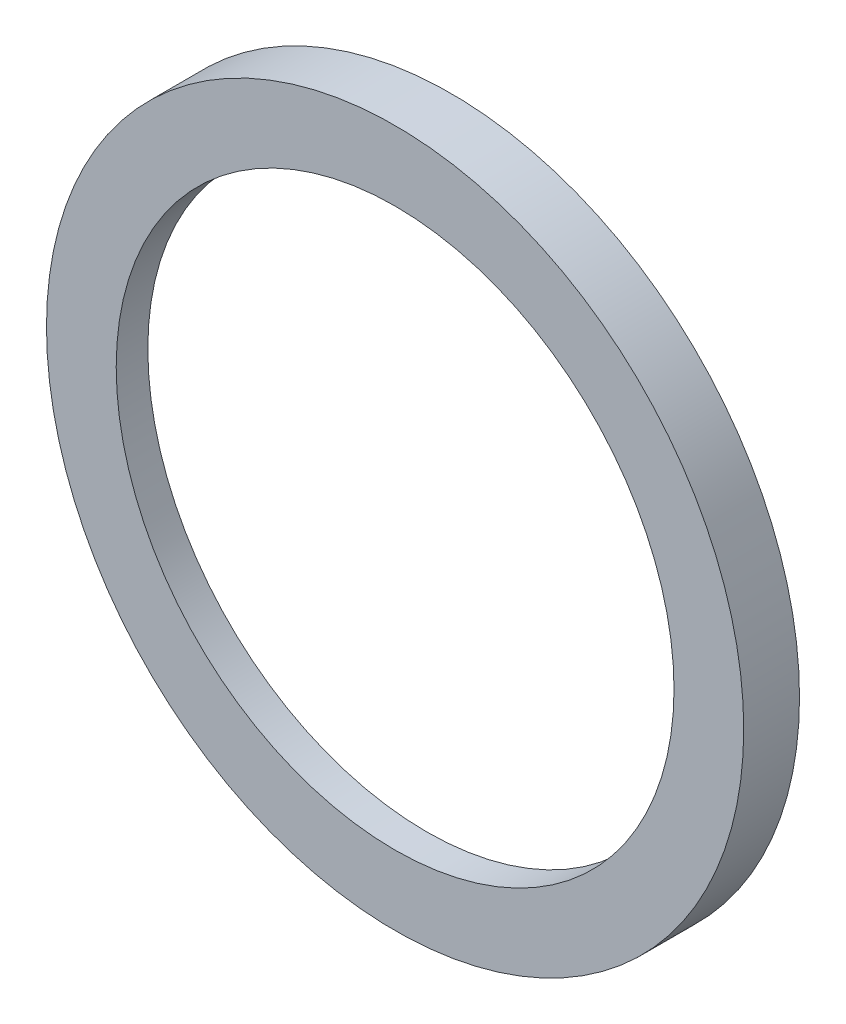
SolidWorks part; units mm, degrees
material "Q235"
ref_plane "Front Plane" through (0, 0, 0) normal (0, 0, 1) x (1, 0, 0)
ref_plane "Top Plane" through (0, 0, 0) normal (0, 1, 0) x (1, 0, 0)
ref_plane "Right Plane" through (0, 0, 0) normal (1, 0, 0) x (0, 0, -1)
sketch "Sketch1" plane through (0, 0, 0) normal (1, 0, 0) x (0, 0, -1)
  line L0 (0, 0) -> (30, 0) construction
  line L1 (0, 150) -> (0, 187.5)
  line L2 (0, 187.5) -> (30, 187.5)
  line L3 (30, 187.5) -> (30, 176)
  line L4 (30, 176) -> (17, 176)
  line L5 (17, 176) -> (17, 150)
  line L6 (17, 150) -> (0, 150)
  dimension "D1" = 30
  dimension "D2" = 13
  dimension "D3" = 375
  dimension "D4" = 352
  dimension "D5" = 300
revolve "Revolve1" add sketch "Sketch1" angle 360 about L0
hole_wizard "M8 Tapped Hole1" positions "Sketch3" profile "Sketch4" tap size "M8" standard "GB"
sketch "Sketch3" plane through (0, 0, -17) normal (0, 0, -1) x (-1, 0, 0)
  point P0 (0, 162.5)
  point P10 (95.5151, 131.4653)
  point P11 (154.5467, 50.2153)
  point P12 (154.5467, -50.2153)
  point P13 (95.5151, -131.4653)
  point P14 (0, -162.5)
  point P15 (-95.5151, -131.4653)
  point P16 (-154.5467, -50.2153)
  point P17 (-154.5467, 50.2153)
  point P18 (-95.5151, 131.4653)
  dimension "D1" = 162.5
  dimension "D2" = 10
sketch "Sketch4" plane through (0, 162.5, -17) normal (1, 0, 0) x (0, 1, 0)
  line L0 (0, 0) -> (0, 13)
  line L1 (0, 13) -> (3.4, 10.9571)
  line L2 (3.4, 10.9571) -> (3.4, 0)
  line L5 (3.4, 0) -> (0, 0)
  line L10 (0, 13) -> (-3.4, 10.9571) construction
  line L11 (0, -6.35) -> (0, 107.95) construction
  dimension "螺纹孔钻头直径" = 6.8
  dimension "螺纹孔钻头深度" = 13
  dimension "导头角度" = 118
cosmetic thread "Hole Cosmetic Thread1" parameters "D1"=10, "D2"=8
cosmetic thread "Hole Cosmetic Thread2" parameters "D1"=10, "D2"=8
cosmetic thread "Hole Cosmetic Thread3" parameters "D1"=10, "D2"=8
cosmetic thread "Hole Cosmetic Thread4" parameters "D1"=10, "D2"=8
cosmetic thread "Hole Cosmetic Thread5" parameters "D1"=10, "D2"=8
cosmetic thread "Hole Cosmetic Thread6" parameters "D1"=10, "D2"=8
cosmetic thread "Hole Cosmetic Thread7" parameters "D1"=10, "D2"=8
cosmetic thread "Hole Cosmetic Thread8" parameters "D1"=10, "D2"=8
cosmetic thread "Hole Cosmetic Thread9" parameters "D1"=10, "D2"=8
cosmetic thread "Hole Cosmetic Thread10" parameters "D1"=10, "D2"=8
